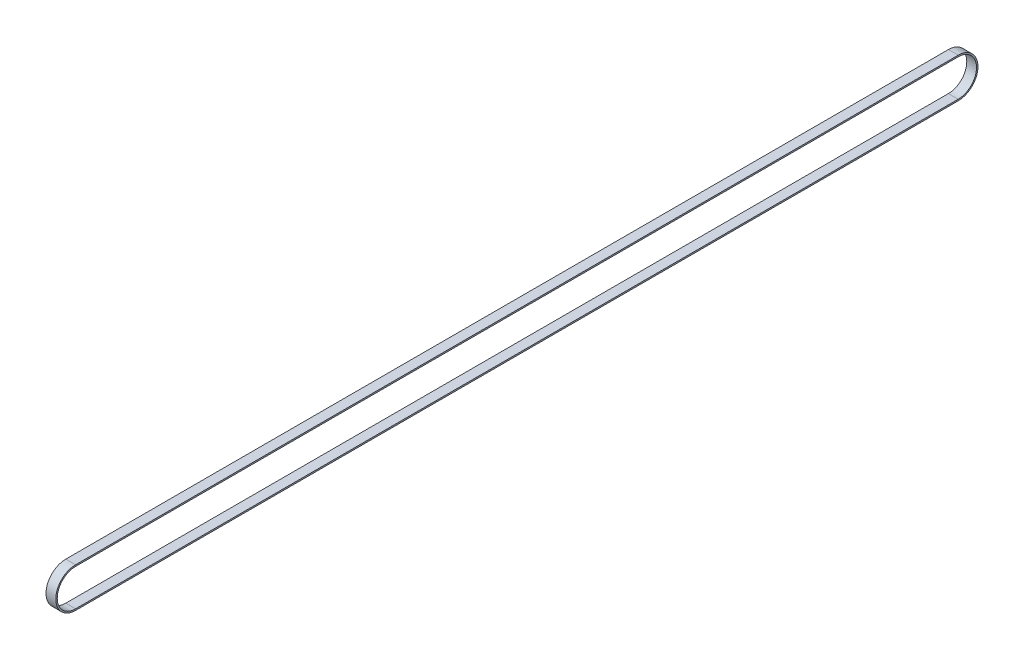
from build123d import *

# Parameters (mm, degrees)
EXTRUDE_1_DEPTH = 15


with BuildPart() as part:
    # 草图2 → 拉伸-薄壁1 (new, symmetric)
    with BuildSketch(Plane(origin=(0, 0, 0), x_dir=(0, 0, -1), z_dir=(1, 0, 0))):
        with BuildLine():
            Line((-2710, -60.795), (0, -60.795))
            ThreePointArc((0, -60.795), (60.795, 0), (0, 60.795))
            Line((0, 60.795), (-2710, 60.795))
            ThreePointArc((-2710, 60.795), (-2770.795, 0), (-2710, -60.795))
        make_face()
        with BuildLine():
            Line((-2710, -56.295), (0, -56.295))
            ThreePointArc((0, -56.295), (56.295, 0), (0, 56.295))
            Line((0, 56.295), (-2710, 56.295))
            ThreePointArc((-2710, 56.295), (-2766.295, 0), (-2710, -56.295))
        make_face(mode=Mode.SUBTRACT)
    extrude(amount=EXTRUDE_1_DEPTH, both=True)


solid = part.part
